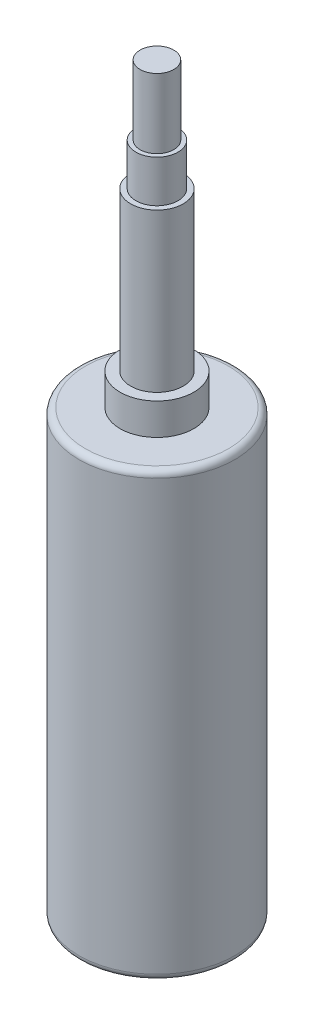
from build123d import *

# Parameters (mm, degrees)
SKETCH_1_R      = 37
EXTRUDE_1_DEPTH = 105
SKETCH_2_R      = 17.5
EXTRUDE_2_DEPTH = 15
SKETCH_3_R      = 12.5
EXTRUDE_3_DEPTH = 75
SKETCH_4_R      = 10
EXTRUDE_4_DEPTH = 20
SKETCH_5_R      = 8
EXTRUDE_5_DEPTH = 33
FILLET_1_R      = 3


with BuildPart() as part:
    # 草图1 → 凸台-拉伸1 (new, symmetric)
    with BuildSketch(Plane(origin=(0, 0, 0), x_dir=(1, 0, 0), z_dir=(0, 1, 0))):
        with Locations(Location((0, 0, 0), (0, 0, 270))):
            Circle(SKETCH_1_R)
    extrude(amount=EXTRUDE_1_DEPTH, both=True)

    # 草图2 → 凸台-拉伸2 (add)
    with BuildSketch(Plane(origin=(0, 105, 0), x_dir=(1, 0, 0), z_dir=(0, 1, 0))):
        with Locations(Location((0, 0, 0), (0, 0, 270))):
            Circle(SKETCH_2_R)
    extrude(amount=EXTRUDE_2_DEPTH)

    # 草图3 → 凸台-拉伸3 (add)
    with BuildSketch(Plane(origin=(0, 120, 0), x_dir=(1, 0, 0), z_dir=(0, 1, 0))):
        with Locations(Location((0, 0, 0), (0, 0, 270))):
            Circle(SKETCH_3_R)
    extrude(amount=EXTRUDE_3_DEPTH)

    # 草图4 → 凸台-拉伸4 (add)
    with BuildSketch(Plane(origin=(0, 195, 0), x_dir=(1, 0, 0), z_dir=(0, 1, 0))):
        with Locations(Location((0, 0, 0), (0, 0, 270))):
            Circle(SKETCH_4_R)
    extrude(amount=EXTRUDE_4_DEPTH)

    # 草图5 → 凸台-拉伸5 (add)
    with BuildSketch(Plane(origin=(0, 215, 0), x_dir=(1, 0, 0), z_dir=(0, 1, 0))):
        with Locations(Location((0, 0, 0), (0, 0, 270))):
            Circle(SKETCH_5_R)
    extrude(amount=EXTRUDE_5_DEPTH)

    # 圆角1
    fillet_1_edges = [part.edges().sort_by_distance(p)[0] for p in [
        (0, -105, -37),
        (0, 105, -37),
    ]]
    fillet(fillet_1_edges, radius=FILLET_1_R)


solid = part.part
